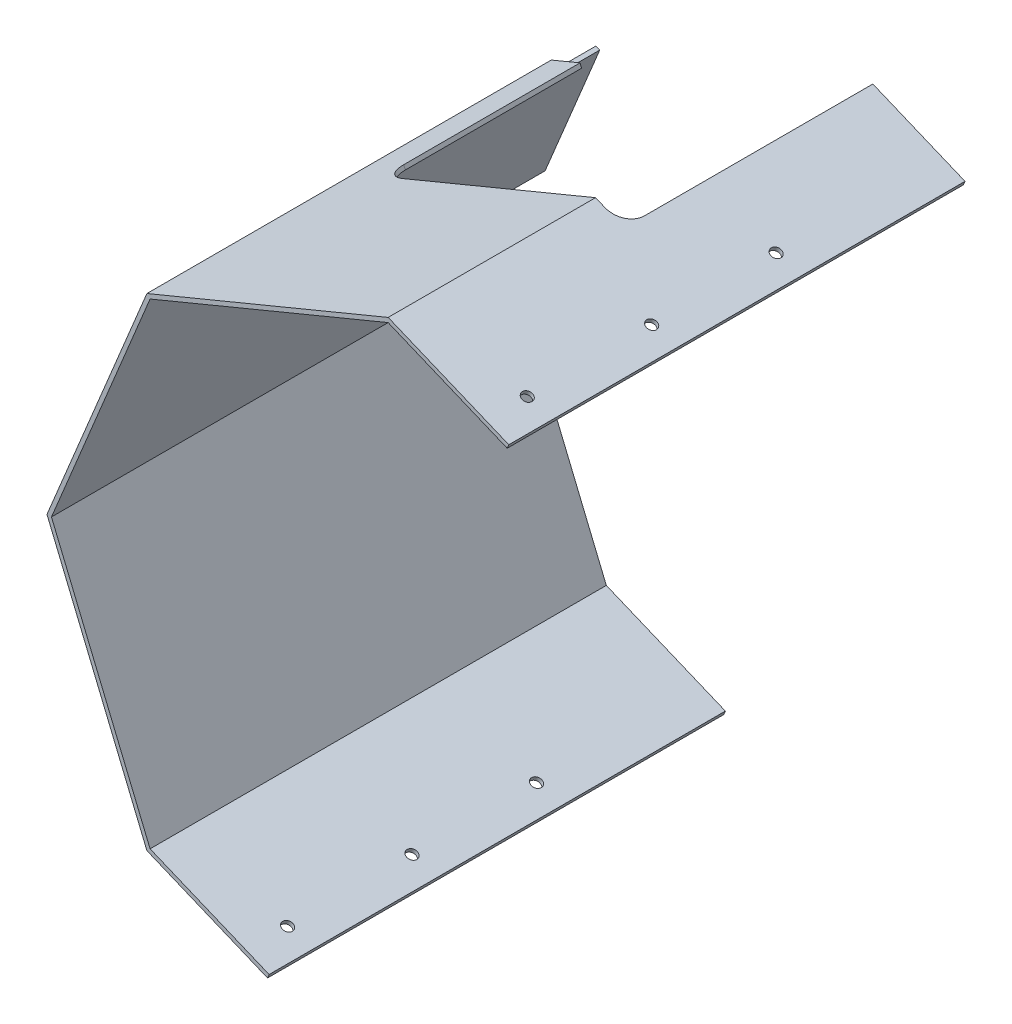
from build123d import *

# Parameters (mm, degrees)
BOSS_EXTRUDE1_DEPTH = 220
SHELL1_T            = -2
CUT_EXTRUDE1_DEPTH  = 321.212491043
SKETCH3_R           = 2.5
CUT_EXTRUDE2_DEPTH  = 394.612153142
SKETCH4_W           = 120
SKETCH4_H           = 120
CUT_EXTRUDE3_DEPTH  = 376.254580252
CUT_EXTRUDE4_DEPTH  = 120
FILLET1_R           = 10
CUT_EXTRUDE5_REACH  = 377.255
SKETCH6_W           = 20
SKETCH6_H           = 25
CUT_EXTRUDE6_DEPTH  = 25
FILLET2_R           = 5
SKETCH8_W           = 20
SKETCH8_H           = 52
CUT_EXTRUDE7_DEPTH  = 357.766015962
CUT_EXTRUDE8_DEPTH  = 20
FILLET3_R           = 5


with BuildPart() as part:
    # Sketch1 → Boss-Extrude1 (new body)
    with BuildSketch(Plane.XY):
        Polygon((-164.523614444, 0), (-116.335763439, -116.335763439), (0, -164.523614444), (116.335763439, -116.335763439), (164.523614444, 0), (116.335763439, 116.335763439), (0, 164.523614444), (-116.335763439, 116.335763439), align=None)
    extrude(amount=BOSS_EXTRUDE1_DEPTH)

    # Shell1
    shell1_openings = [part.faces().sort_by_distance(p)[0] for p in [
        (0, 0, 220),
        (0, 0, 0),
    ]]
    offset(amount=SHELL1_T, openings=shell1_openings, kind=Kind.INTERSECTION)

    # Sketch2 → Cut-Extrude1 (cut, through all)
    with BuildSketch(Plane.XY.offset(220)):
        Polygon((75.61693775, 182.555436661), (-82.042454152, -198.068005503), (95.714298716, -271.697263345), (253.373690618, 108.92617882), align=None)
    extrude(amount=-CUT_EXTRUDE1_DEPTH, mode=Mode.SUBTRACT)

    # Sketch3 → Cut-Extrude2 (cut, through all)
    with BuildSketch(Plane(origin=(-58.167881719, -140.429688942, 0), x_dir=(0.9238795325112961, -0.3826834323650676, 0), z_dir=(-0.3826834323650675, -0.923879532511296, 0))):
        with Locations((-12, 200)):
            Circle(SKETCH3_R)
        with Locations((-12, 140)):
            Circle(SKETCH3_R)
        with Locations((-12, 80)):
            Circle(SKETCH3_R)
    extrude(amount=-CUT_EXTRUDE2_DEPTH, mode=Mode.SUBTRACT)

    # Sketch4 → Cut-Extrude3 (cut, through all)
    with BuildSketch(Plane(origin=(-58.167881719, 140.429688942, 0), x_dir=(0.9238795325112777, 0.3826834323651116, 0), z_dir=(-0.38268343236511165, 0.9238795325112779, 0))):
        with Locations((12.039538519, -60)):
            Rectangle(SKETCH4_W, SKETCH4_H)
    extrude(amount=-CUT_EXTRUDE3_DEPTH, mode=Mode.SUBTRACT)

    # Sketch5 → Cut-Extrude4 (cut)
    with BuildSketch(Plane(origin=(0, 0, 0), x_dir=(-1, 0, 0), z_dir=(0, 0, -1))):
        Polygon((-12.944778014, 156.996927428), (-11.862385814, 159.610053358), (-13.710144879, 158.844686494), align=None)
    extrude(amount=-CUT_EXTRUDE4_DEPTH, mode=Mode.SUBTRACT)

    # Fillet1
    fillet1_edges = [part.edges().sort_by_distance(p)[0] for p in [
        (-102.094887019, 121.152135392, 120),
        (13.327461447, 157.920806961, 120),
    ]]
    fillet(fillet1_edges, radius=FILLET1_R)

    # Sketch6 → Cut-Extrude5 (cut, up to next)
    with BuildSketch(Plane(origin=(-58.167881719, 140.429688942, 0), x_dir=(0.9238795325112777, 0.3826834323651116, 0), z_dir=(-0.38268343236511165, 0.9238795325112779, 0)), mode=Mode.PRIVATE) as cut_extrude5_sk1:
        with Locations((-57.960461481, -12.5)):
            Rectangle(SKETCH6_W, SKETCH6_H)
    cut_extrude5_tool1 = extrude(cut_extrude5_sk1.sketch, amount=-CUT_EXTRUDE5_REACH, mode=Mode.PRIVATE) & part.part
    add(cut_extrude5_tool1.solids().sort_by_distance((-111.716366, 118.249181, 12.5))[0], mode=Mode.SUBTRACT)

    # Sketch7 → Cut-Extrude6 (cut)
    with BuildSketch(Plane(origin=(0, 0, 0), x_dir=(-1, 0, 0), z_dir=(0, 0, -1))):
        Polygon((117.959351739, 107.189822685), (119.04174394, 109.802948615), (119.807110804, 107.95518955), align=None)
    extrude(amount=-CUT_EXTRUDE6_DEPTH, mode=Mode.SUBTRACT)

    # Fillet2
    fillet2_edges = [part.edges().sort_by_distance(p)[0] for p in [
        (-118.883231272, 107.572506117, 25),
    ]]
    fillet(fillet2_edges, radius=FILLET2_R)

    # Sketch8 → Cut-Extrude7 (cut, through all)
    with BuildSketch(Plane(origin=(-140.429688942, 58.167881719, 0), x_dir=(0, 0, 1), z_dir=(-0.9238795325112957, 0.3826834323650681, 0))):
        with Locations((10, -40.960461481)):
            Rectangle(SKETCH8_W, SKETCH8_H)
    extrude(amount=-CUT_EXTRUDE7_DEPTH, mode=Mode.SUBTRACT)

    # Sketch9 → Cut-Extrude8 (cut)
    with BuildSketch(Plane(origin=(0, 0, 0), x_dir=(-1, 0, 0), z_dir=(0, 0, -1))):
        Polygon((159.745704114, -6.30864406), (161.593463179, -7.074010925), (162.358830044, -5.22625186), align=None)
    extrude(amount=-CUT_EXTRUDE8_DEPTH, mode=Mode.SUBTRACT)

    # Fillet3
    fillet3_edges = [part.edges().sort_by_distance(p)[0] for p in [
        (-145.230930158, 43.963534128, 20),
        (-160.669583647, -6.691327492, 20),
    ]]
    fillet(fillet3_edges, radius=FILLET3_R)


solid = part.part
